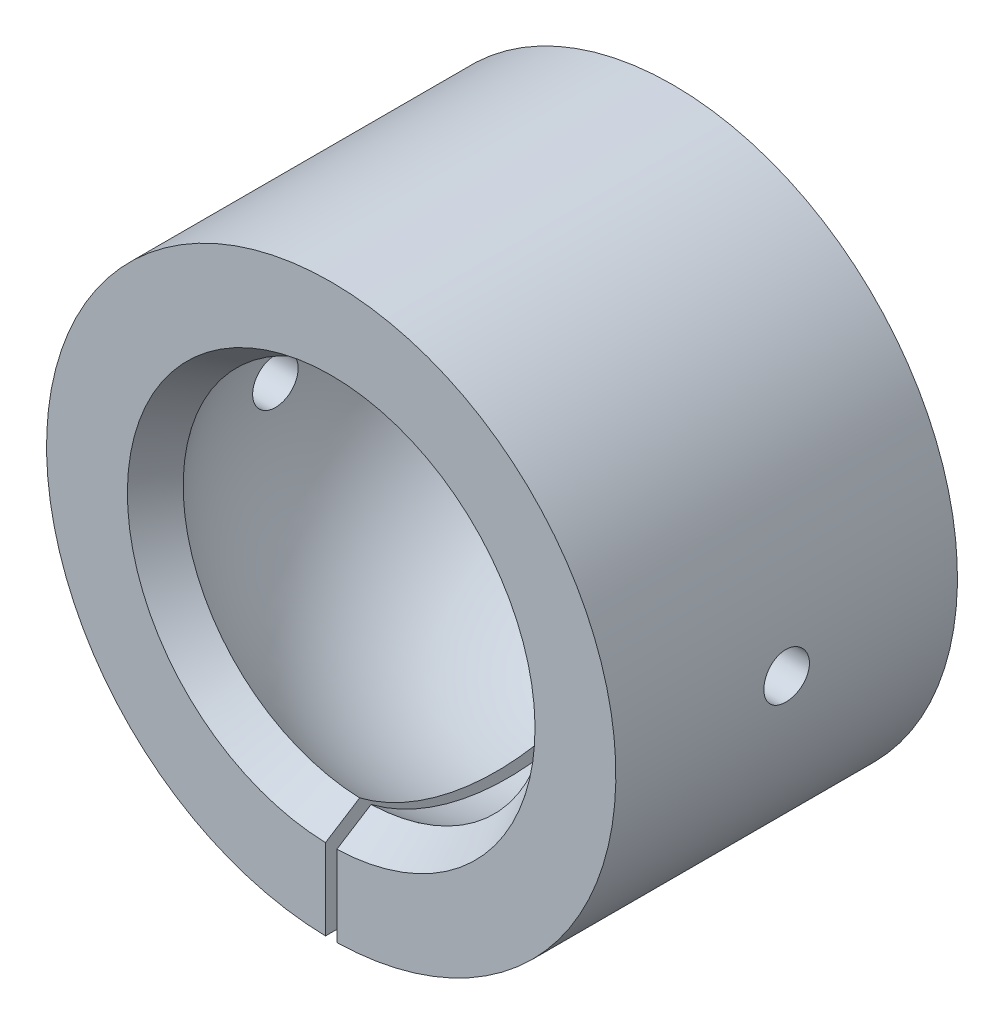
from build123d import *

# Parameters (mm, degrees)
SKETCH_2_W               = 1
SKETCH_2_H               = 35
CUT_EXTRUDE_1_DEPTH      = 39.405728739
CUT_EXTRUDE_2_DEPTH      = 39.405728739
CUT_EXTRUDE_2_DEPTH_BACK = 39.405728739
SKETCH_3_R               = 2


with BuildPart() as part:
    # 草图1 → 旋转1 (revolve)
    with BuildSketch(Plane(origin=(0, 0, 0), x_dir=(1, 0, 0), z_dir=(0, 1, 0))):
        with BuildLine():
            Line((17.9, -15), (16, -12))
            ThreePointArc((16, -12), (19.895478191, 2.042044945), (13.228756555, 15))
            Line((13.228756555, 15), (25, 15))
            Line((25, 15), (25, -15))
            Line((25, -15), (17.9, -15))
        make_face()
    revolve(axis=Axis((0, 0, -23.629385965), (0, 0, 1)))

    # 草图2 → 切除-拉伸1 (cut, through all)
    with BuildSketch(Plane(origin=(0, 0, 0), x_dir=(1, 0, 0), z_dir=(0, 1, 0))):
        Rectangle(SKETCH_2_W, SKETCH_2_H)
    extrude(amount=-CUT_EXTRUDE_1_DEPTH, mode=Mode.SUBTRACT)

    # 草图3 → 切除-拉伸2 (cut, two sides: drawn at the far end of the back side and taken through both)
    with BuildSketch(Plane(origin=(0, 0, 0), x_dir=(0, 0, -1), z_dir=(1, 0, 0)).offset(-CUT_EXTRUDE_2_DEPTH_BACK)):
        Circle(SKETCH_3_R)
    extrude(amount=CUT_EXTRUDE_2_DEPTH + CUT_EXTRUDE_2_DEPTH_BACK, mode=Mode.SUBTRACT)


solid = part.part
